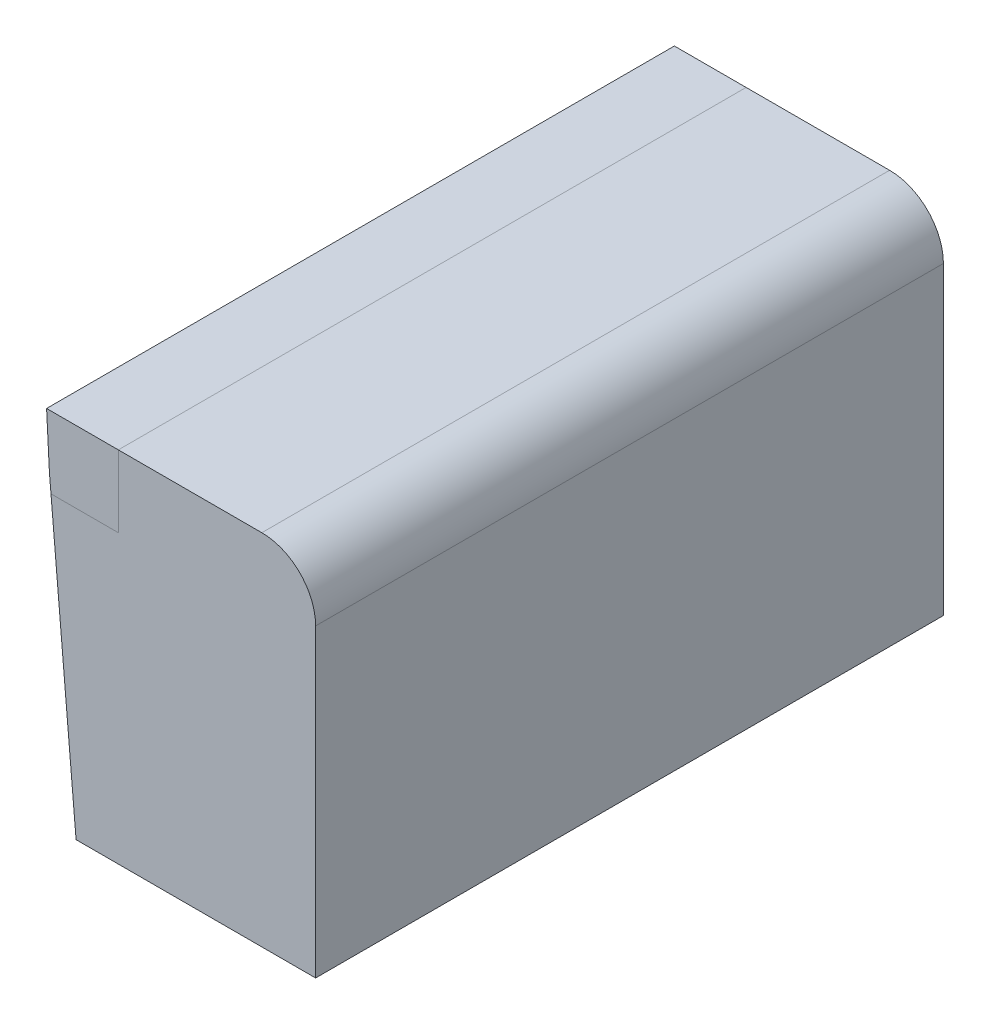
from build123d import *

# Parameters (mm, degrees)
BOSS_EXTRUDE1_DEPTH        = 17.5
SPLIT1_SURFACE_1_BACK      = 44.012
SPLIT1_SURFACE_1_DEPTH     = 88.024
SPLIT1_SURFACE_2_BACK      = 44.012
SPLIT1_SURFACE_2_DEPTH     = 88.024
M6_TAPPED_HOLE1_AT_2_COUNT = 2
M6_TAPPED_HOLE1_AT_2_PITCH = 20
FILLET1_R                  = 3


with BuildPart() as part:
    # Sketch1 → Boss-Extrude1 (new, symmetric)
    with BuildSketch(Plane.XY):
        Polygon((-14.842776662, 17), (-15, 20), (0, 20), (0, 0), (-13.355469382, 0), align=None)
    extrude(amount=BOSS_EXTRUDE1_DEPTH, both=True)


with BuildPart() as body_2:
    # Split1: the piece behind the surface
    add(part.part)
    # Split1 surface: a surface, the sketch's curves swept straight by 88.024 mm
    with BuildLine(Plane.XY.offset(17.5).offset(-SPLIT1_SURFACE_1_BACK), mode=Mode.PRIVATE) as split1_surface_1_path:
        Line((-15, 20), (-11, 20))
        Line((-11, 20), (-11, 16))
        Line((-11, 16), (-15, 16))
        Line((-15, 16), (-15, 20))
    split1_surface_1 = Shell.extrude(split1_surface_1_path.wire(), (0 * SPLIT1_SURFACE_1_DEPTH, 0 * SPLIT1_SURFACE_1_DEPTH, 1 * SPLIT1_SURFACE_1_DEPTH))
    split(bisect_by=split1_surface_1, keep=Keep.BOTTOM)


with BuildPart() as part_1:
    add(part.part)

    # Split1: split by a surface, the side it looks to stays
    # Split1 surface: a surface, the sketch's curves swept straight by 88.024 mm
    with BuildLine(Plane.XY.offset(17.5).offset(-SPLIT1_SURFACE_2_BACK), mode=Mode.PRIVATE) as split1_surface_2_path:
        Line((-15, 20), (-11, 20))
        Line((-11, 20), (-11, 16))
        Line((-11, 16), (-15, 16))
        Line((-15, 16), (-15, 20))
    split1_surface_2 = Shell.extrude(split1_surface_2_path.wire(), (0 * SPLIT1_SURFACE_2_DEPTH, 0 * SPLIT1_SURFACE_2_DEPTH, 1 * SPLIT1_SURFACE_2_DEPTH))
    split(bisect_by=split1_surface_2, keep=Keep.TOP)

    # Sketch3 → M6 Tapped Hole1 (revolve, cut)
    with BuildSketch(Plane(origin=(-6, 0, 10), x_dir=(0, 0, -1), z_dir=(1, 0, 0))):
        Polygon((0, 0), (0, 16.502151548), (2.5, 15), (2.5, 0), align=None)
    m6_tapped_hole1 = revolve(axis=Axis((-6, -6.35, 10), (0, 1, 0)), mode=Mode.SUBTRACT)

    # M6 Tapped Hole1 at 2: M6 Tapped Hole1 ×2
    with Locations(*[(0, 0, -i * M6_TAPPED_HOLE1_AT_2_PITCH) for i in range(1, M6_TAPPED_HOLE1_AT_2_COUNT)]):
        add(m6_tapped_hole1, mode=Mode.SUBTRACT)

    # Fillet1
    fillet1_edges = [part_1.edges().sort_by_distance(p)[0] for p in [
        (0, 20, 0),
    ]]
    fillet(fillet1_edges, radius=FILLET1_R)


solid = Compound([body_2.part, part_1.part])
